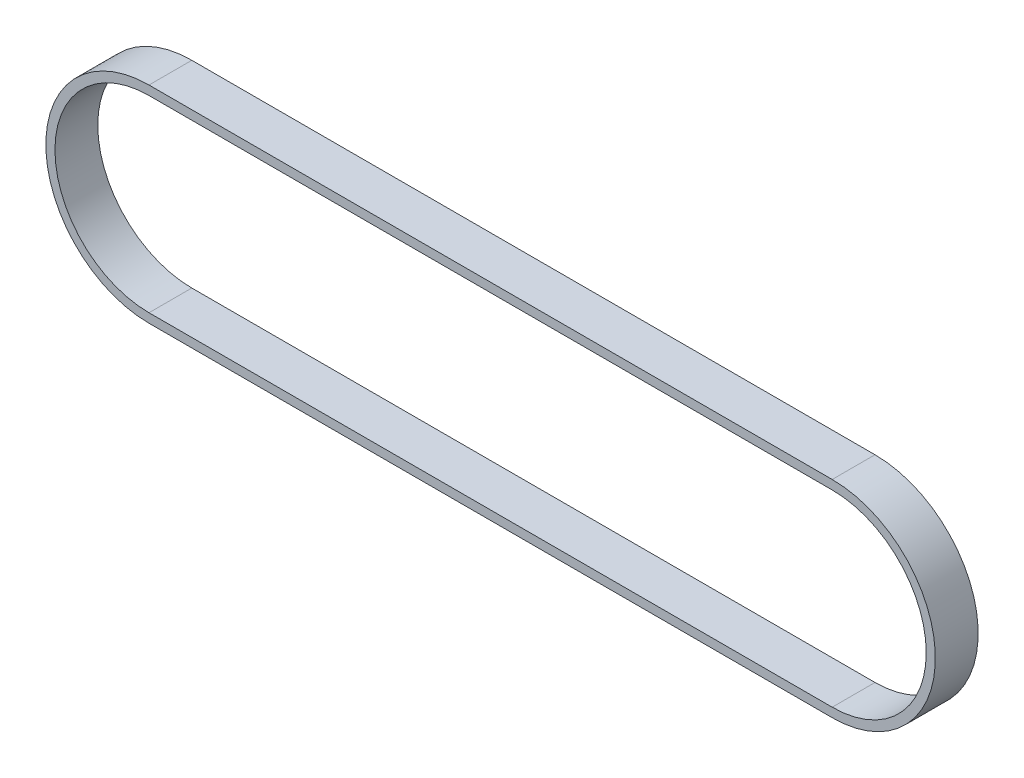
from build123d import *

# Parameters (mm, degrees)
EXTRUDE_1_DEPTH = 4.7


with BuildPart() as part:
    # 草图1 → 拉伸-薄壁1 (new, symmetric)
    with BuildSketch(Plane.XY):
        with BuildLine():
            Line((150, -22.65), (0, -22.65))
            ThreePointArc((0, -22.65), (-22.65, 0), (0, 22.65))
            Line((0, 22.65), (150, 22.65))
            ThreePointArc((150, 22.65), (172.65, 0), (150, -22.65))
        make_face()
        with BuildLine():
            Line((150, -20.65), (0, -20.65))
            ThreePointArc((0, -20.65), (-20.65, 0), (0, 20.65))
            Line((0, 20.65), (150, 20.65))
            ThreePointArc((150, 20.65), (170.65, 0), (150, -20.65))
        make_face(mode=Mode.SUBTRACT)
    extrude(amount=EXTRUDE_1_DEPTH, both=True)


solid = part.part
